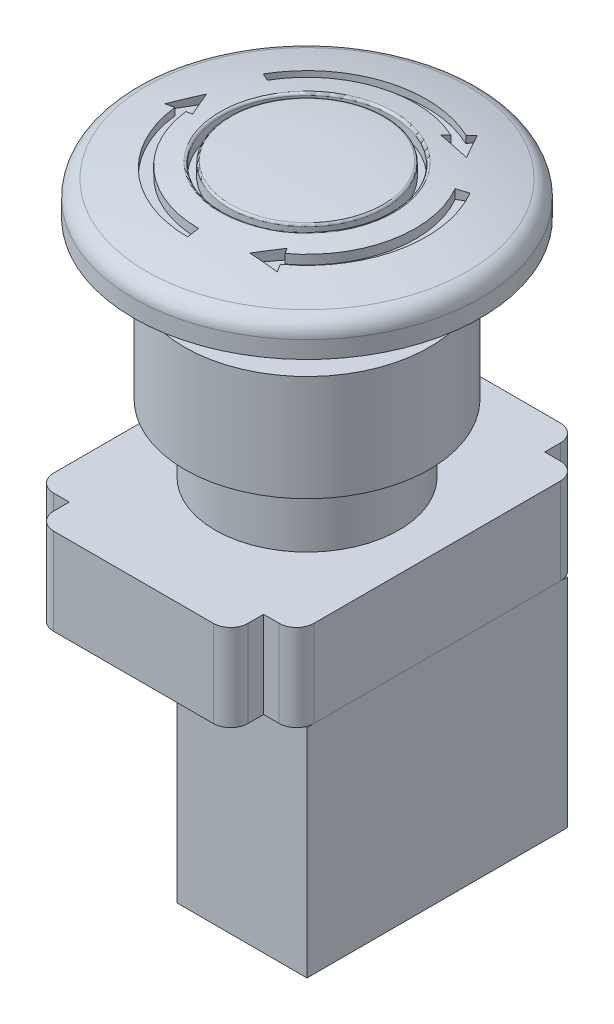
SolidWorks part; units mm, degrees
ref_plane "前视基准面" through (0, 0, 0) normal (0, 0, 1) x (1, 0, 0)
ref_plane "上视基准面" through (0, 0, 0) normal (0, 1, 0) x (1, 0, 0)
ref_plane "右视基准面" through (0, 0, 0) normal (1, 0, 0) x (0, 0, -1)
sketch "草图1" plane through (0, 0, 0) normal (0, 0, 1) x (1, 0, 0)
  line L0 (0, 0) -> (0, 32) construction
  line L1 (14.1, 20) -> (11, 20)
  line L2 (14.1, 20) -> (14.1, 7.8)
  line L3 (14.1, 7.8) -> (10.6, 7.8)
  line L4 (10.6, 7.8) -> (10.6, 0)
  line L5 (10.6, 0) -> (0, 0)
  line L6 (0, 0) -> (0, 32)
  line L7 (11, 20) -> (11, 29)
  line L9 (20, 29.3713) -> (20, 25.8713)
  line L10 (20, 25.8713) -> (18.5381, 25.8713)
  line L11 (18.5381, 25.8713) -> (18.5381, 27.3886)
  arc A0 (18.5381, 27.3886) -> (11, 29) centre (0.3589, -39.2149) ccw
  arc A1 (0, 32) -> (20, 29.3713) centre (1.142, -36.7083) cw
  dimension "D1" = 21.2
  dimension "D2" = 28.2
  dimension "D3" = 7.8
  dimension "D4" = 3.5
  dimension "D5" = 9
revolve "旋转1" add sketch "草图1" angle 360 about L0
sketch "草图2" plane through (0, 0, 0) normal (0, -1, 0) x (1, 0, 0)
  line L0 (15, -20) -> (-15, 20) construction
  line L1 (15, 20) -> (-15, 20)
  line L2 (15, 20) -> (15, -20)
  line L3 (15, -20) -> (-15, -20)
  line L4 (-15, 20) -> (-15, -20)
  dimension "D1" = 30
  dimension "D2" = 40
extrude "拉伸1" add sketch "草图2" along normal blind 10 separate body
sketch "草图3" plane through (0, -10, 0) normal (0, -1, 0) x (1, 0, 0)
  line L0 (15, -20) -> (15, 20) construction
  line L1 (15, 15) -> (0, 15)
  line L2 (15, 15) -> (15, -15)
  line L3 (15, -15) -> (0, -15)
  line L4 (0, 15) -> (0, -15)
  dimension "D1" = 30
extrude "拉伸2" add sketch "草图3" along normal blind 25 separate body
sketch "草图7" plane through (0, 0, 0) normal (0, 1, 0) x (-1, 0, 0)
  line L0 (0, 20) -> (0, -20) construction
  line L1 (-15, 20) -> (-11.2, 20)
  line L2 (-15, 20) -> (-15, 16.2)
  line L3 (-15, 16.2) -> (-11.2, 16.2)
  line L4 (-11.2, 20) -> (-11.2, 16.2)
  line L5 (-15, 20) -> (15, 20) construction
  line L6 (15, -20) -> (-15, -20) construction
  line L7 (-15, 0) -> (15, 0) construction
  line L8 (-15, -20) -> (-15, 20) construction
  line L9 (15, 20) -> (15, -20) construction
  line L10 (11.2, 20) -> (11.2, 16.2)
  line L11 (15, 16.2) -> (11.2, 16.2)
  line L12 (15, 20) -> (15, 16.2)
  line L13 (15, 20) -> (11.2, 20)
  line L14 (15, -20) -> (11.2, -20)
  line L15 (15, -20) -> (15, -16.2)
  line L16 (15, -16.2) -> (11.2, -16.2)
  line L17 (11.2, -20) -> (11.2, -16.2)
  line L18 (-11.2, -20) -> (-11.2, -16.2)
  line L19 (-15, -16.2) -> (-11.2, -16.2)
  line L20 (-15, -20) -> (-15, -16.2)
  line L21 (-15, -20) -> (-11.2, -20)
  dimension "D1" = 3.8
extrude "切除-拉伸2" cut sketch "草图7" against normal up to next (10 mm away)
fillet "圆角1" radius 2 8 edges at (-15, -5, 16.2) (-11.2, -5, 20) (11.2, -5, 20) (15, -5, 16.2) (15, -5, -16.2) (11.2, -5, -20) (-11.2, -5, -20) (-15, -5, -16.2)
fillet "圆角2" radius 2 1 edges at (0, 29.3713, -20)
ref_plane "基准面1" through (0, 30, 0) normal (0, 1, 0) x (-1, 0, 0)
sketch "草图8" plane through (0, 30, 0) normal (0, 1, 0) x (-1, 0, 0)
  circle A0 centre (0, 0) radius 9
  circle A1 centre (0, 0) radius 9.75
  dimension "D1" = 18
  dimension "D2" = 19.5
extrude "切除-拉伸4" cut sketch "草图8" along normal blind 5
sketch "草图9" plane through (0, 30, 0) normal (0, 1, 0) x (-1, 0, 0)
  line L0 (0, 0) -> (12.3616, 0) construction
  line L1 (11.9078, -6.875) -> (10.8253, -6.25)
  line L2 (0, 0) -> (14.4144, -8.3221) construction
  line L3 (0, 12.5) -> (0, 13.75)
  line L4 (14.8368, 1.5631) -> (13.0558, -1.4734)
  line L5 (-10.8253, -6.25) -> (-11.9078, -6.875)
  line L6 (-8.4786, 11.9078) -> (-5.3338, 11.9078)
  line L7 (-5.3338, 11.9078) -> (-7.1941, 9.4669)
  line L8 (-7.1941, 9.4669) -> (-7.4818, 10.0136)
  line L9 (-8.0705, 11.1324) -> (-8.4786, 11.9078)
  line L10 (13.6609, 1.5631) -> (14.8368, 1.5631)
  line L11 (13.0558, -1.4734) -> (11.6251, 1.5631)
  line L12 (11.6251, 1.5631) -> (12.4019, 1.5631)
  line L13 (-6.3905, -13.2364) -> (-8.2704, -10.1084)
  line L14 (-8.2704, -10.1084) -> (-4.7726, -10.6477)
  line L15 (-4.7726, -10.6477) -> (-5.2173, -11.3591)
  line L17 (-5.8847, -12.4271) -> (-6.3905, -13.2364)
  arc A0 (-7.4818, 10.0136) -> (-10.8253, -6.25) centre (0, 0) ccw
  arc A1 (-8.0705, 11.1324) -> (-11.9078, -6.875) centre (0, 0) ccw
  arc A2 (-5.2173, -11.3591) -> (10.8253, -6.25) centre (0, 0) ccw
  arc A3 (-5.8847, -12.4271) -> (11.9078, -6.875) centre (0, 0) ccw
  arc A4 (13.6609, 1.5631) -> (0, 13.75) centre (0, 0) ccw
  arc A5 (12.4019, 1.5631) -> (0, 12.5) centre (0, 0) ccw
  dimension "D1" = 25
  dimension "D2" = 27.5
  dimension "D3" = 90
  dimension "D4" = 30
extrude "切除-拉伸5" cut sketch "草图9" along normal blind 5
fillet "圆角3" radius 0.25 2 edges at (0, 31.4682, -9.75) (0, 31.5587, -9)
